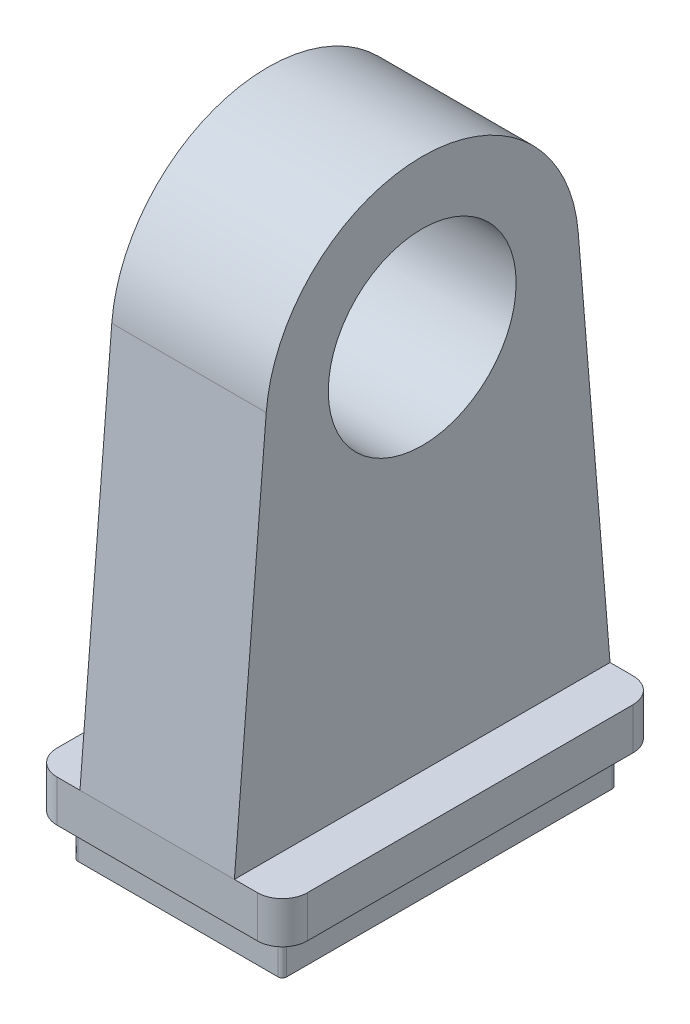
SolidWorks part; units mm, degrees
ref_plane "Front Plane" through (0, 0, 0) normal (0, 0, 1) x (1, 0, 0)
ref_plane "Top Plane" through (0, 0, 0) normal (0, 1, 0) x (1, 0, 0)
ref_plane "Right Plane" through (0, 0, 0) normal (1, 0, 0) x (0, 0, -1)
sketch "Sketch 1" plane through (0, 0, 0) normal (0, 1, 0) x (1, 0, 0)
  line L0 (0, 180.7895) -> (0, -186.3158) construction
  line L1 (-167.3684, 0) -> (124.7368, 0) construction
  line L2 (48, 90) -> (-48, 90)
  line L3 (-60, 78) -> (-60, -78)
  line L4 (60, 78) -> (60, -78)
  line L5 (48, -90) -> (-48, -90)
  arc A0 (-48, 90) -> (-60, 78) centre (-48, 78) ccw
  arc A1 (48, 90) -> (60, 78) centre (48, 78) cw
  arc A2 (48, -90) -> (60, -78) centre (48, -78) ccw
  arc A3 (-48, -90) -> (-60, -78) centre (-48, -78) cw
  point P8 (0, -90)
  point P13 (-60, 0)
  point P14 (0, 90)
  point P20 (60, 0)
  dimension "D3" = 12
  dimension "D1" = 120
  dimension "D2" = 180
extrude "Boss-Extrude 1" add sketch "Sketch 1" along normal blind 20
sketch "Sketch 2" plane through (0, 0, 0) normal (0, -1, 0) x (1, 0, 0)
  line L8 (-48, -80) -> (48, -80)
  line L9 (50, -78) -> (50, 78)
  line L10 (48, 80) -> (-48, 80)
  line L11 (-50, 78) -> (-50, -78)
  line L12 (-48, -80) -> (48, -80)
  line L13 (50, -78) -> (50, 78)
  line L14 (48, 80) -> (-48, 80)
  line L15 (-50, 78) -> (-50, -78)
  arc A8 (-50, -78) -> (-48, -80) centre (-48, -78) ccw
  arc A9 (48, -80) -> (50, -78) centre (48, -78) ccw
  arc A10 (50, 78) -> (48, 80) centre (48, 78) ccw
  arc A11 (-48, 80) -> (-50, 78) centre (-48, 78) ccw
  arc A12 (-50, -78) -> (-48, -80) centre (-48, -78) ccw
  arc A13 (48, -80) -> (50, -78) centre (48, -78) ccw
  arc A14 (50, 78) -> (48, 80) centre (48, 78) ccw
  arc A15 (-48, 80) -> (-50, 78) centre (-48, 78) ccw
  dimension "D1" = 10
extrude "Boss-Extrude 2" add sketch "Sketch 2" along normal blind 20
sketch "Sketch 3" plane through (0, 0, 0) normal (1, 0, 0) x (0, 0, -1)
  line L0 (0, 313.4651) -> (0, -36.5781) construction
  line L2 (78, 0) -> (-78, 0) construction
  line L3 (-74.7495, 206.1247) -> (-90, 20)
  line L4 (-90, 20) -> (90, 20)
  line L5 (-78, 20) -> (78, 20) construction
  line L6 (74.7495, 206.1247) -> (90, 20)
  arc A0 (74.7495, 206.1247) -> (-74.7495, 206.1247) centre (0, 200) ccw
  circle A1 centre (0, 200) radius 45
  point P14 (0, 20)
  dimension "D1" = 200
  dimension "D2" = 90
  dimension "D3" = 75
extrude "Boss-Extrude 3" add sketch "Sketch 3" along normal mid plane 74
